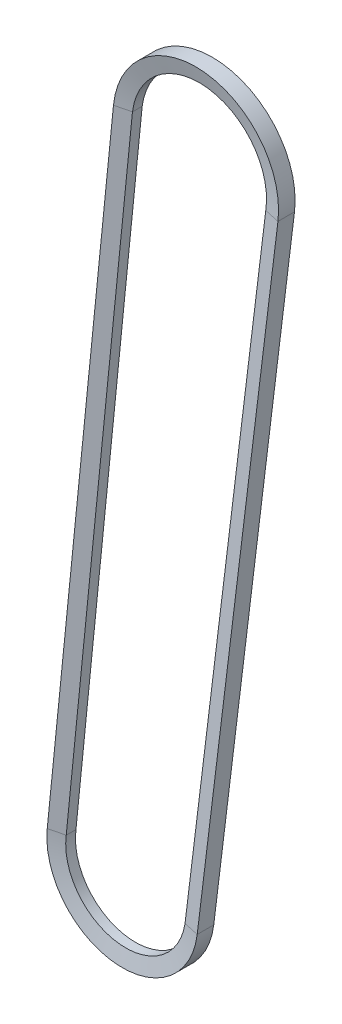
SolidWorks part; units mm, degrees
ref_plane "前视基准面" through (0, 0, 0) normal (0, 0, 1) x (1, 0, 0)
ref_plane "上视基准面" through (0, 0, 0) normal (0, 1, 0) x (1, 0, 0)
ref_plane "右视基准面" through (0, 0, 0) normal (1, 0, 0) x (0, 0, -1)
other "Configuration Table"
sketch "草图1" plane through (0, 0, 0) normal (0, 0, 1) x (1, 0, 0)
  line L0 (133.935, 322.9682) -> (50.9909, -352.7994)
  line L1 (-35.0064, 341.8177) -> (-103.0439, -335.6131)
  arc A0 (133.935, 322.9682) -> (-35.0064, 341.8177) centre (49.5681, 333.3234) ccw
  arc A1 (-103.0439, -335.6131) -> (50.9909, -352.7994) centre (-25.9319, -343.3579) ccw
  dimension "D1" = 170
  dimension "D2" = 155
  dimension "D3" = 68.9896
  dimension "D4" = 336.9889
  dimension "D5" = 675.7676
  dimension "D6" = 677.4308
ref_plane "基准面1" through (0, 322.9682, 0) normal (0, 1, 0) x (1, 0, 0)
sketch "草图2" plane through (0, 322.9682, 0) normal (0, 1, 0) x (1, 0, 0)
  line L0 (133.935, 8.5) -> (133.935, -8.5)
  line L1 (133.935, -8.5) -> (117.935, -5)
  line L2 (117.935, -5) -> (117.935, 5)
  line L3 (-35.0064, 0) -> (134.5681, 0) construction
  line L4 (133.935, 0) -> (117.935, 0) construction
  line L5 (133.935, 8.5) -> (117.935, 5)
  dimension "D1" = 8.5
  dimension "D2" = 5
  dimension "D3" = 16
sweep "扫描1" add profiles "草图2" path "草图1"
